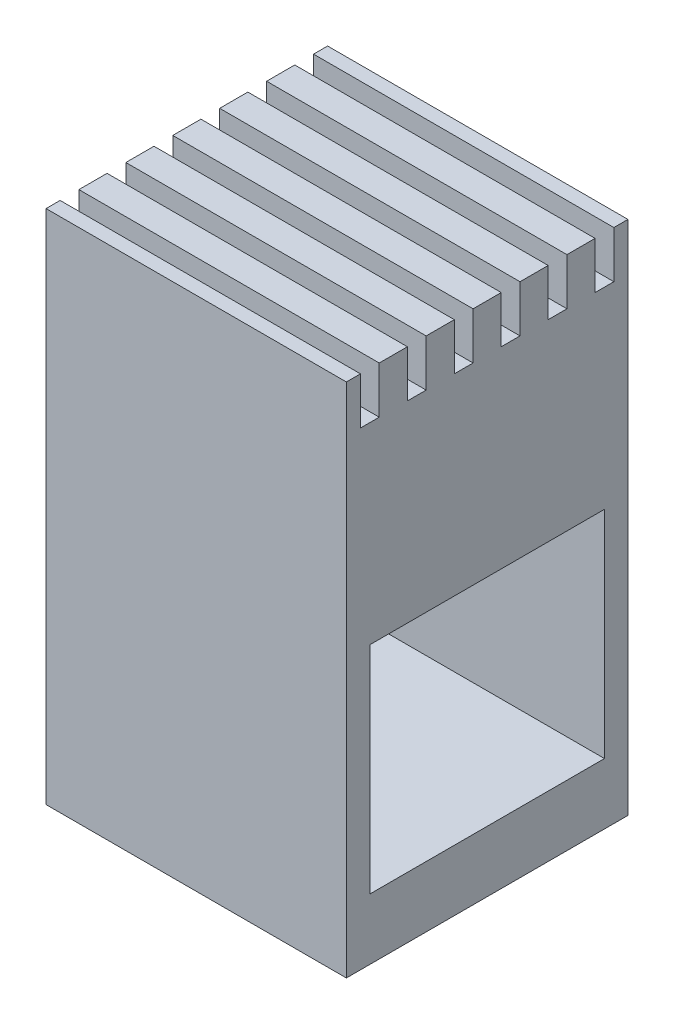
from build123d import *

# Parameters (mm, degrees)
SKETCH_1_W             = 32
SKETCH_1_H             = 30
EXTRUDE_1_DEPTH        = 55
HOLE_WIZARD_M3_1_D     = 2.5
HOLE_WIZARD_M3_1_DEPTH = 7.5
HOLE_WIZARD_M3_1_TIP   = 0.751075774
SKETCH_5_W             = 25
SKETCH_5_H             = 23
CUT_EXTRUDE_2_DEPTH    = 60
SKETCH_6_W             = 2
SKETCH_6_H             = 5
CUT_EXTRUDE_3_DEPTH    = 66.375836515
PATTERN_LINEAR_1_COUNT = 6
PATTERN_LINEAR_1_PITCH = 5


with BuildPart() as part:
    # 草图1 → 凸台-拉伸1 (new body)
    with BuildSketch(Plane(origin=(0, 0, 0), x_dir=(1, 0, 0), z_dir=(0, 1, 0))):
        Rectangle(SKETCH_1_W, SKETCH_1_H)
    extrude(amount=EXTRUDE_1_DEPTH)

    # M3 螺纹孔1
    with Locations(Plane(origin=(0, 0, 0), x_dir=(-1, 0, 0), z_dir=(0, -1, 0))):
        with Locations((9, 7.5), (9, -7.5)):
            Hole(HOLE_WIZARD_M3_1_D / 2, depth=HOLE_WIZARD_M3_1_DEPTH)
            with Locations((0, 0, -(HOLE_WIZARD_M3_1_DEPTH + HOLE_WIZARD_M3_1_TIP / 2))):  # 118° drill point
                Cone(0, HOLE_WIZARD_M3_1_D / 2, HOLE_WIZARD_M3_1_TIP, mode=Mode.SUBTRACT)

    # 草图5 → 切除-拉伸2 (cut)
    with BuildSketch(Plane(origin=(16, 0, 0), x_dir=(0, 0, -1), z_dir=(1, 0, 0))):
        with Locations((0, 18)):
            Rectangle(SKETCH_5_W, SKETCH_5_H)
    extrude(amount=-CUT_EXTRUDE_2_DEPTH, mode=Mode.SUBTRACT)

    # 草图6 → 切除-拉伸3 (cut, through all)
    with BuildSketch(Plane(origin=(16, 0, 0), x_dir=(0, 0, -1), z_dir=(1, 0, 0))):
        with Locations((-12.5, 52.5)):
            Rectangle(SKETCH_6_W, SKETCH_6_H)
    cut_extrude_3 = extrude(amount=-CUT_EXTRUDE_3_DEPTH, mode=Mode.SUBTRACT)

    # 阵列(线性)1: 切除-拉伸3 ×6
    with Locations(*[(0, 0, -i * PATTERN_LINEAR_1_PITCH) for i in range(1, PATTERN_LINEAR_1_COUNT)]):
        add(cut_extrude_3, mode=Mode.SUBTRACT)


solid = part.part
